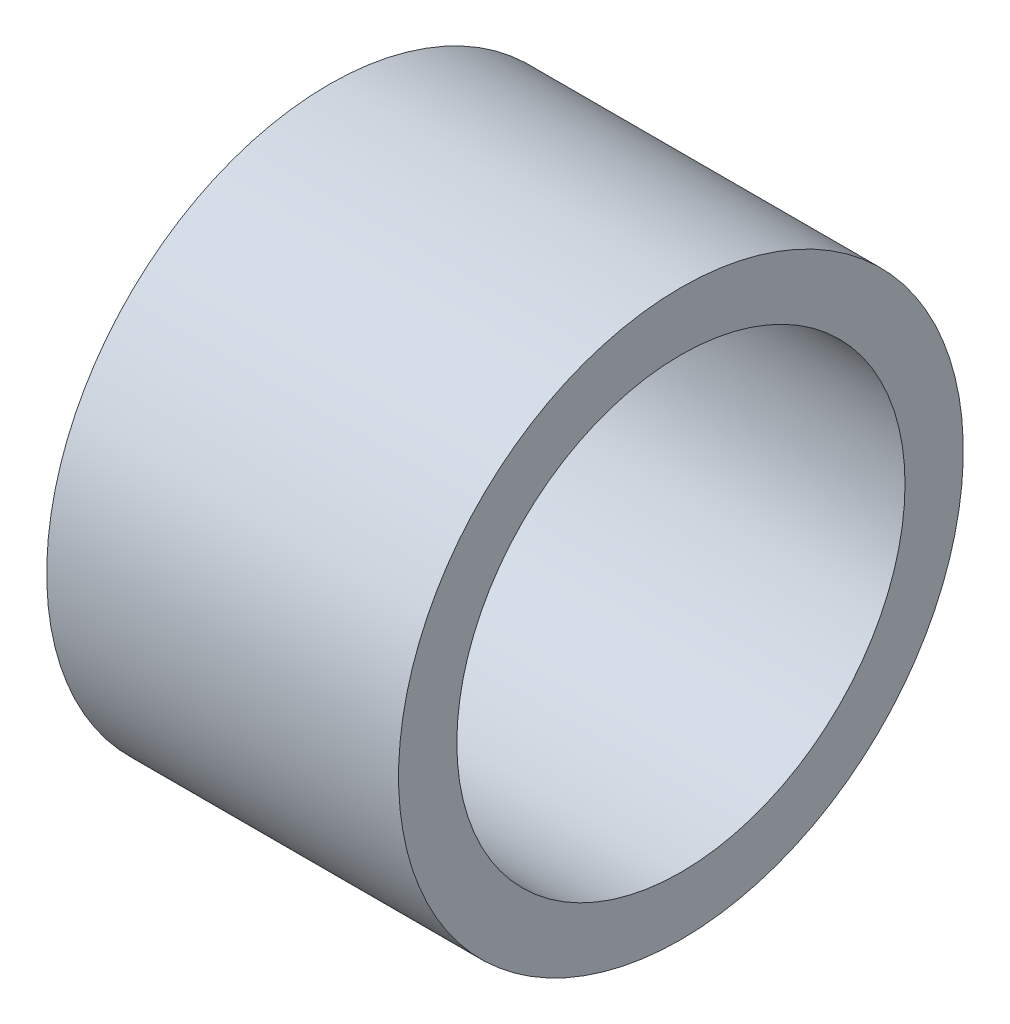
SolidWorks part; units mm, degrees
ref_plane "Front Plane" through (0, 0, 0) normal (0, 0, 1) x (1, 0, 0)
ref_plane "Top Plane" through (0, 0, 0) normal (0, 1, 0) x (1, 0, 0)
ref_plane "Right Plane" through (0, 0, 0) normal (1, 0, 0) x (0, 0, -1)
other "Configuration Table"
sketch "Sketch1" plane through (191.75, 0, 0) normal (1, 0, 0) x (0, 0, -1)
  circle A0 centre (102.5, 90) radius 31.5
  circle A1 centre (102.5, 90) radius 25
  dimension "D1" = 50
  dimension "D2" = 63
extrude "Boss-Extrude1" add sketch "Sketch1" along normal blind 39.25
